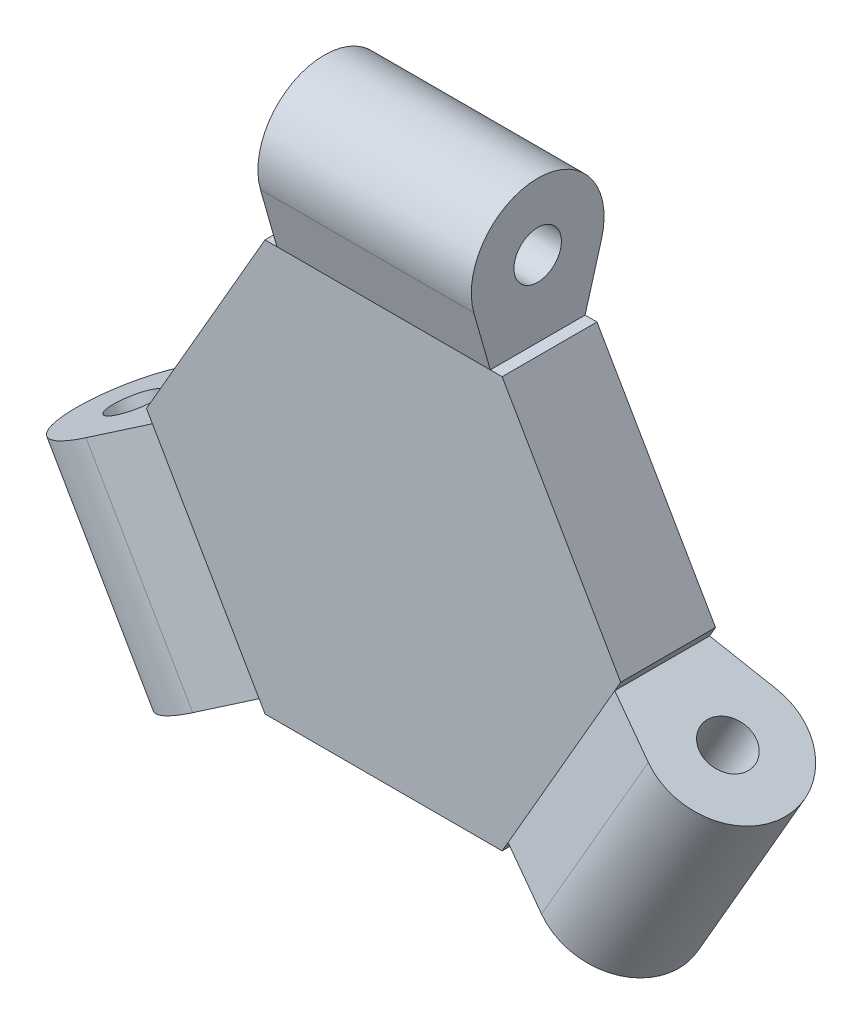
from build123d import *

# Parameters (mm, degrees)
BOSS_EXTRUDE1_DEPTH = 20
SKETCH2_R           = 5
BOSS_EXTRUDE2_DEPTH = 22.5
SKETCH4_R           = 5
CUT_EXTRUDE1_DEPTH  = 0.5
CIRPATTERN1_COUNT   = 3


with BuildPart() as part:
    # Sketch1 → Boss-Extrude1 (new body)
    with BuildSketch(Plane.XY):
        Polygon((50, 0), (25, 43.301270189), (-25, 43.301270189), (-50, 0), (-25, -43.301270189), (25, -43.301270189), align=None)
    extrude(amount=BOSS_EXTRUDE1_DEPTH)

    # Sketch2 → Boss-Extrude2 (add, symmetric)
    with BuildSketch(Plane(origin=(0, 0, 0), x_dir=(0, 0, -1), z_dir=(1, 0, 0))):
        with BuildLine():
            Line((-20, 43.301270189), (-23.46513086, 55.465896517))
            ThreePointArc((-23.46513086, 55.465896517), (-10.001520995, 73.301270167), (3.464086976, 55.467405029))
            Line((3.464086976, 55.467405029), (0, 43.301270189))
            Line((0, 43.301270189), (-20, 43.301270189))
        make_face()
        with Locations(Location((-10.000736748, 59.301270189, 0), (0, 0, 180))):
            Circle(SKETCH2_R, mode=Mode.SUBTRACT)
    boss_extrude2 = extrude(amount=BOSS_EXTRUDE2_DEPTH, both=True)

    # Sketch4 → Cut-Extrude1 (cut)
    with BuildSketch(Plane(origin=(0, 0, 0), x_dir=(-1, 0, 0), z_dir=(0, 0, -1))):
        Circle(SKETCH4_R)
    extrude(amount=-CUT_EXTRUDE1_DEPTH, mode=Mode.SUBTRACT)

    # CirPattern1: Boss-Extrude2 ×3 about axis
    cirpattern1_axis = Axis((0, 0, 0), (0, 0, 1))
    for i in range(1, CIRPATTERN1_COUNT):
        add(boss_extrude2.rotate(cirpattern1_axis, i * 360 / CIRPATTERN1_COUNT))


solid = part.part
